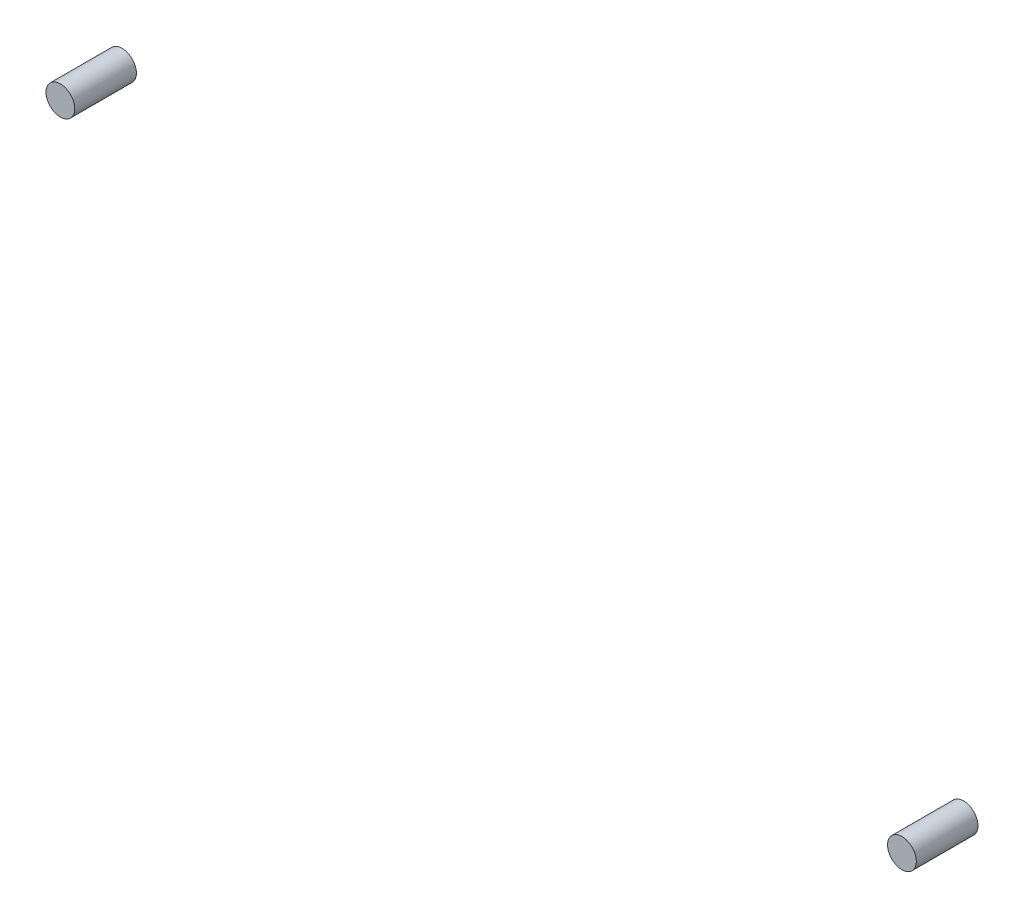
SolidWorks part; units mm, degrees
material "20"
ref_plane "Front Plane" through (0, 0, 0) normal (0, 0, 1) x (1, 0, 0)
ref_plane "Top Plane" through (0, 0, 0) normal (0, 1, 0) x (1, 0, 0)
ref_plane "Right Plane" through (0, 0, 0) normal (1, 0, 0) x (0, 0, -1)
sketch "Sketch1" plane through (0, 0, 0) normal (0, 0, 1) x (1, 0, 0)
  line L0 (609, 460) -> (609, 355) construction
  line L1 (210.5652, 490.2776) -> (210.5652, 494.2776) construction
  circle A0 centre (629, 379.8776) radius 7
  arc A1 (619.8652, 377.8776) -> (637.8652, 377.8776) centre (628.8652, 377.8776) ccw construction
  circle A2 centre (219.5652, 492.2776) radius 7
  arc A3 (210.5652, 490.2776) -> (228.5652, 490.2776) centre (219.5652, 490.2776) ccw construction
  point P7 (628.8652, 368.8776)
  point P15 (219.5652, 481.2776)
  dimension "D1" = 14
  dimension "D2" = 20
  dimension "D3" = 11
  dimension "D4" = 9
  dimension "D6" = 14
  dimension "D5" = 11
extrude "Boss-Extrude1" add sketch "Sketch1" along normal blind 30
